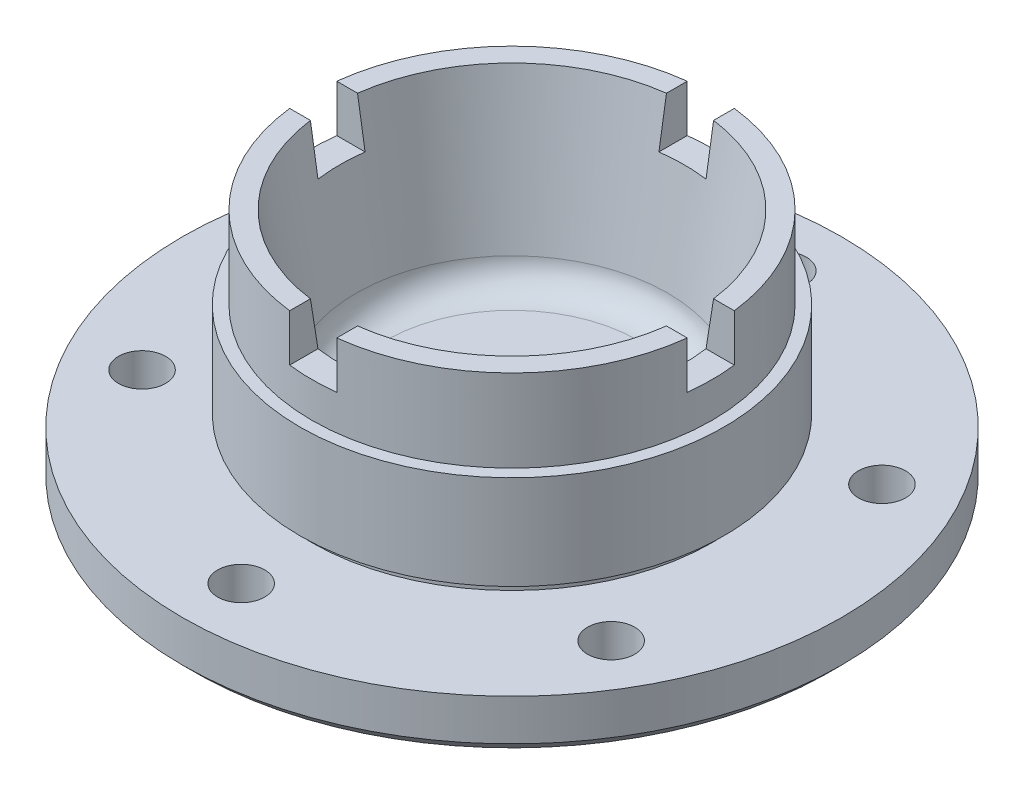
from build123d import *

# Parameters (mm, degrees)
SKETCH2_W          = 33.532576539
SKETCH2_H          = 8
SKETCH2_W_2        = 8
SKETCH2_H_2        = 33.532576539
CUT_EXTRUDE1_DEPTH = 8
SKETCH3_R          = 4
CUT_EXTRUDE2_DEPTH = 94
SCALE_1_SCALE      = 1.875


with BuildPart() as part:
    # Sketch1 → Revolve1 (revolve)
    with BuildSketch(Plane.XY, mode=Mode.PRIVATE) as revolve1_sk:
        with BuildLine():
            Line((0, 11), (0, 2))
            Line((0, 2), (31, 2))
            Line((31, 2), (32, 0))
            Line((32, 0), (54, 0))
            Line((54, 0), (56, 2))
            Line((56, 2), (56, 9))
            Line((56, 9), (34, 9))
            Line((34, 9), (34, 11))
            Line((34, 11), (36, 11))
            Line((36, 11), (36, 27))
            Line((36, 27), (34, 27))
            Line((34, 27), (34, 41))
            Line((34, 41), (30.5, 41))
            Line((30.5, 41), (26.45024814, 15.502481405))
            ThreePointArc((26.45024814, 15.502481405), (24.830088793, 12.292737332), (21.475062189, 11))
            Line((21.475062189, 11), (16.570568921, 11))
            Line((16.570568921, 11), (0, 11))
        make_face()
    revolve(revolve1_sk.sketch.rotate(Axis((0, 2, 0), (0, 1, 0)), 90), axis=Axis((0, 2, 0), (0, 1, 0)))

    # Sketch2 → Cut-Extrude1 (cut)
    with BuildSketch(Plane(origin=(0, 41, 0), x_dir=(1, 0, 0), z_dir=(0, 1, 0))):
        with Locations((31.449191607, 0)):
            Rectangle(SKETCH2_W, SKETCH2_H)
        with Locations((0, 31.449191607)):
            Rectangle(SKETCH2_W_2, SKETCH2_H_2)
        with Locations((0, -31.449191607)):
            Rectangle(SKETCH2_W_2, SKETCH2_H_2)
        with Locations((-31.449191607, 0)):
            Rectangle(SKETCH2_W, SKETCH2_H)
    extrude(amount=-CUT_EXTRUDE1_DEPTH, mode=Mode.SUBTRACT)

    # Sketch3 → Cut-Extrude2 (cut)
    with BuildSketch(Plane(origin=(0, 41, 0), x_dir=(1, 0, 0), z_dir=(0, 1, 0))):
        with Locations(Location((-39.837168574, -23, 0), (0, 0, 270))):
            Circle(SKETCH3_R)
        with Locations(Location((0, 46, 0), (0, 0, 270))):
            Circle(SKETCH3_R)
        with Locations(Location((39.837168574, 23, 0), (0, 0, 270))):
            Circle(SKETCH3_R)
        with Locations(Location((-39.837168574, 23, 0), (0, 0, 270))):
            Circle(SKETCH3_R)
        with Locations(Location((0, -46, 0), (0, 0, 270))):
            Circle(SKETCH3_R)
        with Locations(Location((39.837168574, -23, 0), (0, 0, 270))):
            Circle(SKETCH3_R)
    extrude(amount=-CUT_EXTRUDE2_DEPTH, mode=Mode.SUBTRACT)


with BuildPart() as part_1:
    # Scale 1: scaled about (0, 10.8729077, 0)
    add(part.part.scale(SCALE_1_SCALE).moved(Location((0, -9.513794238, 0))))


solid = part_1.part
